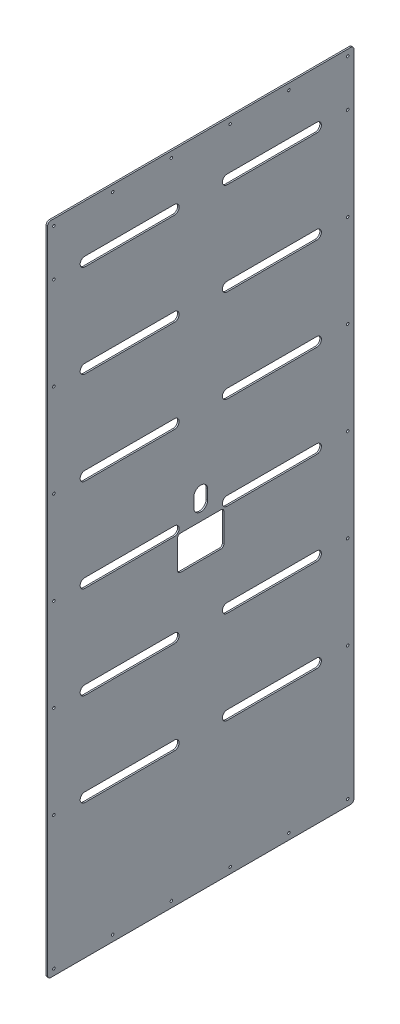
from build123d import *

# Parameters (mm, degrees)
SKETCH1_W                     = 990
SKETCH1_H                     = 2120
BOSS_EXTRUDE1_DEPTH           = 5
FILLET1_R                     = 10
M7_CLEARANCE_HOLE3_D          = 8
M7_CLEARANCE_HOLE2_AT_2_COUNT = 2
M7_CLEARANCE_HOLE2_AT_2_PITCH = 950
LPATTERN7_COUNT               = 6
LPATTERN7_PITCH               = 300
SKETCH16_W                    = 150
SKETCH16_H                    = 110
CUT_EXTRUDE4_DEPTH            = 10
FILLET2_R                     = 10
CUT_EXTRUDE5_DEPTH            = 10
LPATTERN8_COUNT               = 6
LPATTERN8_PITCH               = 300
MIRROR6_COPY_1_DEPTH          = 10
MIRROR6_COPY_2_DEPTH          = 10
MIRROR6_COPY_3_DEPTH          = 10
MIRROR6_COPY_4_DEPTH          = 10
MIRROR6_COPY_5_DEPTH          = 10


with BuildPart() as part:
    # Sketch1 → Boss-Extrude1 (new body)
    with BuildSketch(Plane(origin=(0, 0, 0), x_dir=(0, 0, -1), z_dir=(1, 0, 0))):
        Rectangle(SKETCH1_W, SKETCH1_H)
    extrude(amount=BOSS_EXTRUDE1_DEPTH)

    # Fillet1
    fillet1_edges = [part.edges().sort_by_distance(p)[0] for p in [
        (2.5, -1060, -495),
        (2.5, -1060, 495),
        (2.5, 1060, 495),
        (2.5, 1060, -495),
    ]]
    fillet(fillet1_edges, radius=FILLET1_R)

    # M7 Clearance Hole3 (through all)
    with Locations(Plane(origin=(5, 0, 0), x_dir=(0, 0, -1), z_dir=(1, 0, 0))):
        with Locations((-475, 1040), (-285, 1040), (-95, 1040), (95, 1040), (285, 1040), (475, 1040)):
            m7_clearance_hole3 = Hole(M7_CLEARANCE_HOLE3_D / 2)

    # Mirror5: M7 Clearance Hole3 across plane
    add(m7_clearance_hole3.mirror(Plane(origin=(0, 0, 0), x_dir=(0, 0, 1), z_dir=(0, -1, 0))), mode=Mode.SUBTRACT)

    # Sketch15 → M7 Clearance Hole2 (revolve, cut)
    with BuildSketch(Plane(origin=(5, 890, 475), x_dir=(0, 0, -1), z_dir=(0, 1, 0))):
        Polygon((0, 0), (0, 7.403442476), (4, 5), (4, 0), align=None)
    m7_clearance_hole2 = revolve(axis=Axis((11.35, 890, 475), (-1, 0, 0)), mode=Mode.SUBTRACT)

    # M7 Clearance Hole2 at 2: M7 Clearance Hole2 ×2
    with Locations(*[(0, 0, -i * M7_CLEARANCE_HOLE2_AT_2_PITCH) for i in range(1, M7_CLEARANCE_HOLE2_AT_2_COUNT)]):
        add(m7_clearance_hole2, mode=Mode.SUBTRACT)

    # LPattern7: M7 Clearance Hole2 ×6
    with Locations(*[(0, -i * LPATTERN7_PITCH, 0) for i in range(1, LPATTERN7_COUNT)]):
        add(m7_clearance_hole2, mode=Mode.SUBTRACT)

    # LPattern7 copy 1 sketch → LPattern7 copy 1 (revolve, cut)
    with BuildSketch(Plane(origin=(5, 590, -475), x_dir=(0, 0, -1), z_dir=(0, 1, 0))):
        Polygon((0, 0), (0, 7.403442476), (4, 5), (4, 0), align=None)
    revolve(axis=Axis((11.35, 590, -475), (-1, 0, 0)), mode=Mode.SUBTRACT)

    # LPattern7 copy 2 sketch → LPattern7 copy 2 (revolve, cut)
    with BuildSketch(Plane(origin=(5, 290, -475), x_dir=(0, 0, -1), z_dir=(0, 1, 0))):
        Polygon((0, 0), (0, 7.403442476), (4, 5), (4, 0), align=None)
    revolve(axis=Axis((11.35, 290, -475), (-1, 0, 0)), mode=Mode.SUBTRACT)

    # LPattern7 copy 3 sketch → LPattern7 copy 3 (revolve, cut)
    with BuildSketch(Plane(origin=(5, -10, -475), x_dir=(0, 0, -1), z_dir=(0, 1, 0))):
        Polygon((0, 0), (0, 7.403442476), (4, 5), (4, 0), align=None)
    revolve(axis=Axis((11.35, -10, -475), (-1, 0, 0)), mode=Mode.SUBTRACT)

    # LPattern7 copy 4 sketch → LPattern7 copy 4 (revolve, cut)
    with BuildSketch(Plane(origin=(5, -310, -475), x_dir=(0, 0, -1), z_dir=(0, 1, 0))):
        Polygon((0, 0), (0, 7.403442476), (4, 5), (4, 0), align=None)
    revolve(axis=Axis((11.35, -310, -475), (-1, 0, 0)), mode=Mode.SUBTRACT)

    # LPattern7 copy 5 sketch → LPattern7 copy 5 (revolve, cut)
    with BuildSketch(Plane(origin=(5, -610, -475), x_dir=(0, 0, -1), z_dir=(0, 1, 0))):
        Polygon((0, 0), (0, 7.403442476), (4, 5), (4, 0), align=None)
    revolve(axis=Axis((11.35, -610, -475), (-1, 0, 0)), mode=Mode.SUBTRACT)

    # Sketch16 → Cut-Extrude4 (cut)
    with BuildSketch(Plane(origin=(5, 0, 0), x_dir=(0, 0, -1), z_dir=(1, 0, 0))):
        with BuildLine():
            Line((22.5, 54), (22.5, 24))
            ThreePointArc((22.5, 24), (0, 1.5), (-22.5, 24))
            Line((-22.5, 24), (-22.5, 54))
            ThreePointArc((-22.5, 54), (0, 76.5), (22.5, 54))
        make_face()
        with Locations((0, -80)):
            Rectangle(SKETCH16_W, SKETCH16_H)
    extrude(amount=-CUT_EXTRUDE4_DEPTH, mode=Mode.SUBTRACT)

    # Fillet2
    fillet2_edges = [part.edges().sort_by_distance(p)[0] for p in [
        (2.5, -25, -75),
        (2.5, -135, -75),
        (2.5, -135, 75),
        (2.5, -25, 75),
    ]]
    fillet(fillet2_edges, radius=FILLET2_R)

    # Sketch18 → Cut-Extrude5 (cut)
    with BuildSketch(Plane(origin=(5, 0, 0), x_dir=(0, 0, -1), z_dir=(1, 0, 0))):
        with BuildLine():
            Line((-375, 905), (-85, 905))
            ThreePointArc((-85, 905), (-70, 890), (-85, 875))
            Line((-85, 875), (-375, 875))
            ThreePointArc((-375, 875), (-390, 890), (-375, 905))
        make_face()
    cut_extrude5 = extrude(amount=-CUT_EXTRUDE5_DEPTH, mode=Mode.SUBTRACT)

    # LPattern8: Cut-Extrude5 ×6
    with Locations(*[(0, -i * LPATTERN8_PITCH, 0) for i in range(1, LPATTERN8_COUNT)]):
        add(cut_extrude5, mode=Mode.SUBTRACT)

    # Mirror6: Cut-Extrude5 across plane
    add(cut_extrude5.mirror(Plane.XY), mode=Mode.SUBTRACT)

    # Mirror6 copy 1 sketch → Mirror6 copy 1 (cut)
    with BuildSketch(Plane(origin=(5, -300, 0), x_dir=(0, 0, 1), z_dir=(1, 0, 0))):
        with BuildLine():
            Line((-375, -905), (-85, -905))
            ThreePointArc((-85, -905), (-70, -890), (-85, -875))
            Line((-85, -875), (-375, -875))
            ThreePointArc((-375, -875), (-390, -890), (-375, -905))
        make_face()
    extrude(amount=-MIRROR6_COPY_1_DEPTH, mode=Mode.SUBTRACT)

    # Mirror6 copy 2 sketch → Mirror6 copy 2 (cut)
    with BuildSketch(Plane(origin=(5, -600, 0), x_dir=(0, 0, 1), z_dir=(1, 0, 0))):
        with BuildLine():
            Line((-375, -905), (-85, -905))
            ThreePointArc((-85, -905), (-70, -890), (-85, -875))
            Line((-85, -875), (-375, -875))
            ThreePointArc((-375, -875), (-390, -890), (-375, -905))
        make_face()
    extrude(amount=-MIRROR6_COPY_2_DEPTH, mode=Mode.SUBTRACT)

    # Mirror6 copy 3 sketch → Mirror6 copy 3 (cut)
    with BuildSketch(Plane(origin=(5, -900, 0), x_dir=(0, 0, 1), z_dir=(1, 0, 0))):
        with BuildLine():
            Line((-375, -905), (-85, -905))
            ThreePointArc((-85, -905), (-70, -890), (-85, -875))
            Line((-85, -875), (-375, -875))
            ThreePointArc((-375, -875), (-390, -890), (-375, -905))
        make_face()
    extrude(amount=-MIRROR6_COPY_3_DEPTH, mode=Mode.SUBTRACT)

    # Mirror6 copy 4 sketch → Mirror6 copy 4 (cut)
    with BuildSketch(Plane(origin=(5, -1200, 0), x_dir=(0, 0, 1), z_dir=(1, 0, 0))):
        with BuildLine():
            Line((-375, -905), (-85, -905))
            ThreePointArc((-85, -905), (-70, -890), (-85, -875))
            Line((-85, -875), (-375, -875))
            ThreePointArc((-375, -875), (-390, -890), (-375, -905))
        make_face()
    extrude(amount=-MIRROR6_COPY_4_DEPTH, mode=Mode.SUBTRACT)

    # Mirror6 copy 5 sketch → Mirror6 copy 5 (cut)
    with BuildSketch(Plane(origin=(5, -1500, 0), x_dir=(0, 0, 1), z_dir=(1, 0, 0))):
        with BuildLine():
            Line((-375, -905), (-85, -905))
            ThreePointArc((-85, -905), (-70, -890), (-85, -875))
            Line((-85, -875), (-375, -875))
            ThreePointArc((-375, -875), (-390, -890), (-375, -905))
        make_face()
    extrude(amount=-MIRROR6_COPY_5_DEPTH, mode=Mode.SUBTRACT)


solid = part.part
